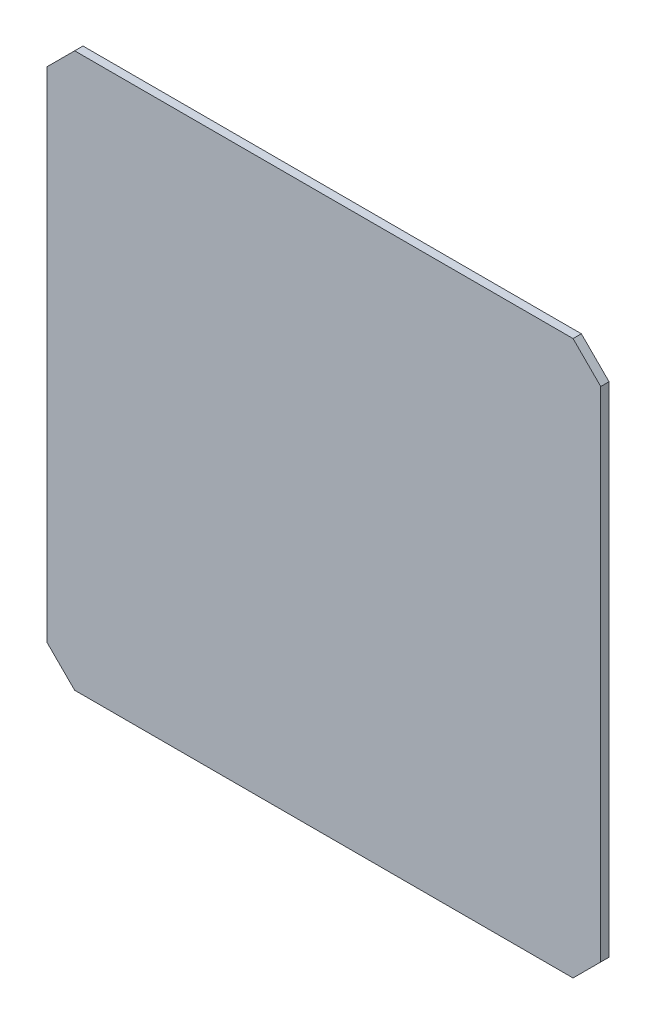
from build123d import *

# Parameters (mm, degrees)
SKETCH_1_W      = 200
SKETCH_1_H      = 200
EXTRUDE_1_DEPTH = 3
CHAMFER_1_SIZE  = 10


with BuildPart() as part:
    # 草图1 → 凸台-拉伸1 (new body)
    with BuildSketch(Plane.XY):
        Rectangle(SKETCH_1_W, SKETCH_1_H)
    extrude(amount=EXTRUDE_1_DEPTH)

    # 倒角1
    chamfer_1_edges = [part.edges().sort_by_distance(p)[0] for p in [
        (100, -100, 1.5),
        (-100, -100, 1.5),
        (-100, 100, 1.5),
        (100, 100, 1.5),
    ]]
    chamfer(chamfer_1_edges, length=CHAMFER_1_SIZE)


solid = part.part
